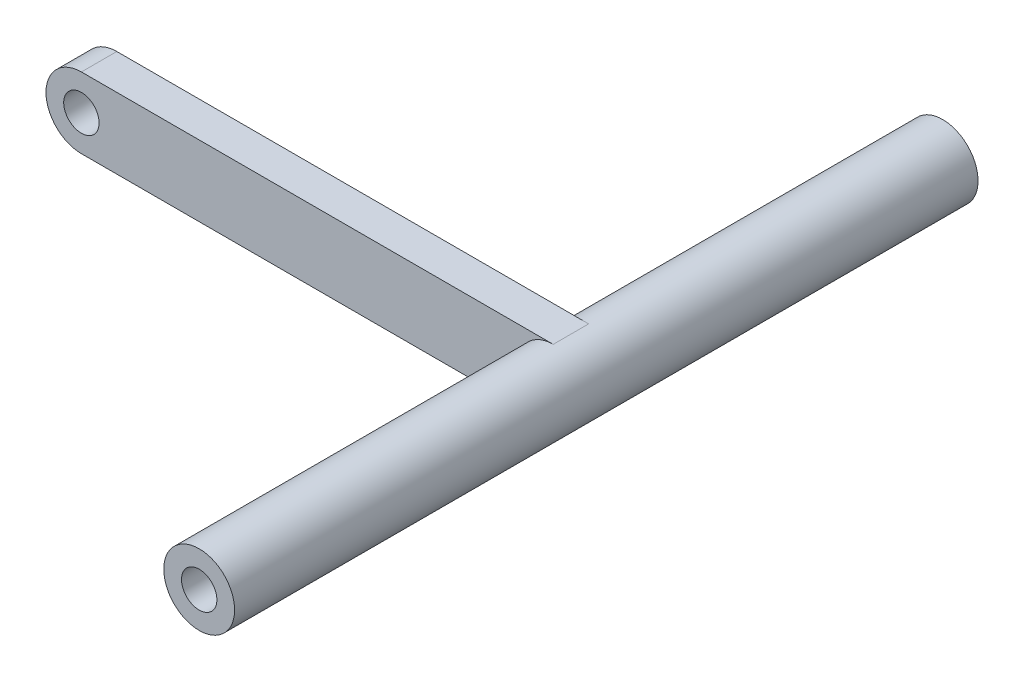
from build123d import *

# Parameters (mm, degrees)
SKETCH_1_R               = 5
SKETCH_1_R_2             = 4.376095709
EXTRUDE_1_DEPTH          = 10
SKETCH_2_R               = 10
EXTRUDE_2_DEPTH          = 100
EXTRUDE_START            = 100
SKETCH_3_R               = 10
EXTRUDE_3_DEPTH          = 100
CUT_EXTRUDE_1_DEPTH      = 224.769799627
CUT_EXTRUDE_1_DEPTH_BACK = 224.769799627
SKETCH_4_R               = 5


with BuildPart() as part:
    # 草图1 → 凸台-拉伸1 (new body)
    with BuildSketch(Plane.XY):
        with BuildLine():
            Line((-66.635, 10), (66.635, 10))
            ThreePointArc((66.635, 10), (76.635, 0), (66.635, -10))
            Line((66.635, -10), (-66.635, -10))
            ThreePointArc((-66.635, -10), (-76.635, 0), (-66.635, 10))
        make_face()
        with Locations((-66.635, 0)):
            Circle(SKETCH_1_R, mode=Mode.SUBTRACT)
        with Locations((66.635, 0)):
            Circle(SKETCH_1_R_2, mode=Mode.SUBTRACT)
    extrude(amount=EXTRUDE_1_DEPTH)

    # 草图2 → 凸台-拉伸2 (add)
    with BuildSketch(Plane.XY.offset(10)):
        with Locations(Location((66.635, 0, 0), (0, 0, 90))):
            Circle(SKETCH_2_R)
    extrude(amount=EXTRUDE_2_DEPTH)

    # 草图3 → 凸台-拉伸3 (add)
    with BuildSketch(Plane(origin=(0, 0, 0), x_dir=(-1, 0, 0), z_dir=(0, 0, -1)).offset(EXTRUDE_START)):
        with Locations((-66.635, 0)):
            Circle(SKETCH_3_R)
    extrude(amount=-EXTRUDE_3_DEPTH)

    # 草图4 → 切除-拉伸1 (cut, two sides: drawn at the far end of the back side and taken through both)
    with BuildSketch(Plane(origin=(0, 0, -100), x_dir=(-1, 0, 0), z_dir=(0, 0, -1)).offset(-CUT_EXTRUDE_1_DEPTH_BACK)):
        with Locations((-66.635, 0)):
            Circle(SKETCH_4_R)
    extrude(amount=CUT_EXTRUDE_1_DEPTH + CUT_EXTRUDE_1_DEPTH_BACK, mode=Mode.SUBTRACT)


solid = part.part
